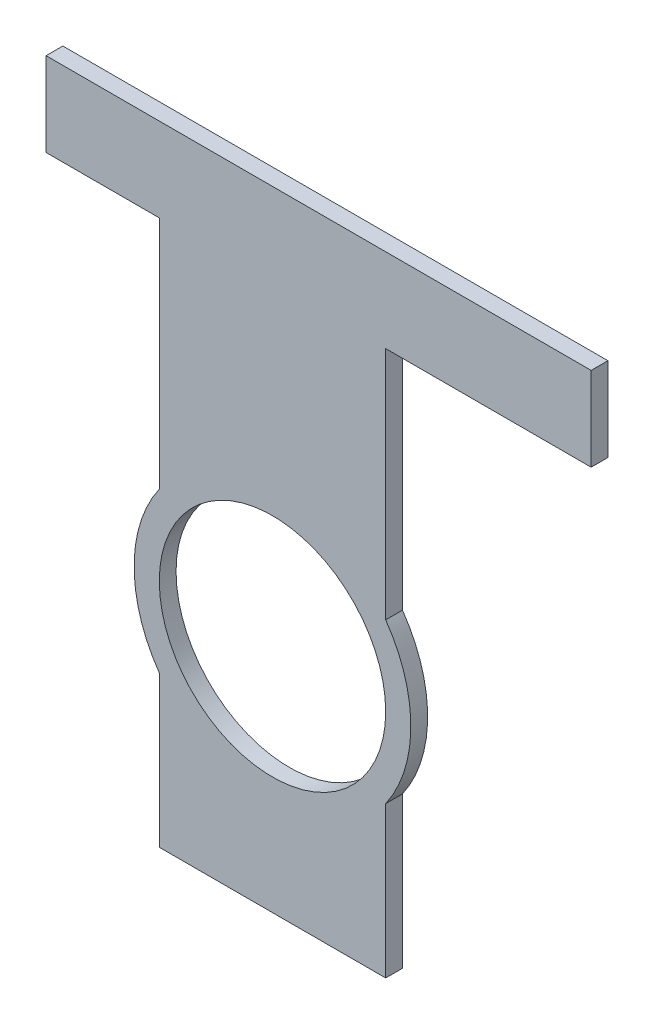
SolidWorks part; units mm, degrees
material "06Cr19Ni10"
ref_plane "Front Plane" through (0, 0, 0) normal (0, 0, 1) x (1, 0, 0)
ref_plane "Top Plane" through (0, 0, 0) normal (0, 1, 0) x (1, 0, 0)
ref_plane "Right Plane" through (0, 0, 0) normal (1, 0, 0) x (0, 0, -1)
sketch "Sketch1" plane through (0, 0, 0) normal (0, 0, 1) x (1, 0, 0)
  line L0 (-135, 475) -> (-135, 94.8683)
  line L1 (135, -475) -> (-135, -475)
  line L2 (135, 475) -> (-135, 475)
  line L5 (0, 300) -> (0, -300) construction
  line L6 (165, 0) -> (-165, 0) construction
  line L7 (135, 475) -> (135, 94.8683)
  line L8 (-135, -475) -> (-135, -94.8683)
  line L9 (135, -475) -> (135, -94.8683)
  arc A0 (-135, 94.8683) -> (-135, -94.8683) centre (0, 0) ccw
  arc A1 (135, -94.8683) -> (135, 94.8683) centre (0, 0) ccw
  circle A2 centre (0, 0) radius 135
  point P0 (0, 0)
  dimension "D3" = 330
  dimension "D2" = 270
  dimension "D1" = 270
extrude "Boss-Extrude2" add sketch "Sketch1" along normal blind 20
sketch "Sketch5" plane through (0, 0, 20) normal (0, 0, 1) x (1, 0, 0)
  line L0 (-135, -94.8683) -> (-135, -475) construction
  line L1 (135, -475) -> (-135, -475)
  line L2 (135, -475) -> (135, -275)
  line L3 (135, -275) -> (-135, -275)
  line L4 (-135, -475) -> (-135, -275)
  dimension "D1" = 200
extrude "Cut-Extrude1" cut sketch "Sketch5" against normal blind 20
sketch "Sketch6" plane through (0, 0, 0) normal (0, 0, -1) x (-1, 0, 0)
  line L0 (0, 475) -> (0, 0) construction
  line L1 (-135, 475) -> (-380, 475)
  line L2 (-135, 475) -> (-135, 375)
  line L3 (-135, 375) -> (-380, 375)
  line L4 (-380, 475) -> (-380, 375)
  line L6 (135, 475) -> (135, 94.8683) construction
  line L7 (135, 475) -> (270, 475)
  line L8 (135, 475) -> (135, 375)
  line L9 (135, 375) -> (270, 375)
  line L10 (270, 475) -> (270, 375)
  dimension "D1" = 100
  dimension "D2" = 380
  dimension "D3" = 270
extrude "Boss-Extrude3" add sketch "Sketch6" against normal blind 20
